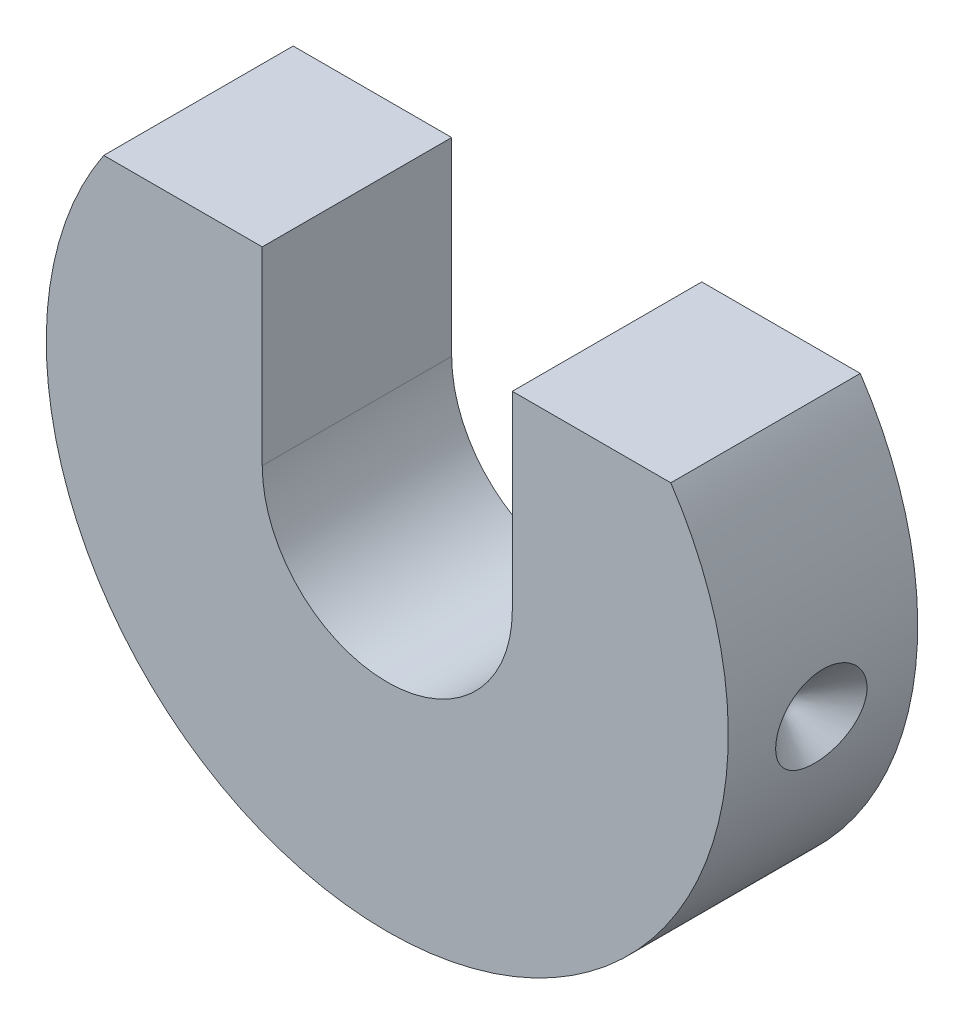
SolidWorks part; units mm, degrees
ref_plane "Front Plane" through (0, 0, 0) normal (0, 0, 1) x (1, 0, 0)
ref_plane "Top Plane" through (0, 0, 0) normal (0, 1, 0) x (1, 0, 0)
ref_plane "Right Plane" through (0, 0, 0) normal (1, 0, 0) x (0, 0, -1)
sketch "Sketch1" plane through (0, 0, 0) normal (0, 0, 1) x (1, 0, 0)
  line L0 (-14.9666, 10) -> (-6.6, 10)
  line L1 (-6.6, 0) -> (-6.6, 10)
  line L2 (6.6, 0) -> (6.6, 10)
  line L3 (6.6, 10) -> (14.9666, 10)
  arc A0 (-14.9666, 10) -> (14.9666, 10) centre (0, 0) ccw
  arc A1 (-6.6, 0) -> (6.6, 0) centre (0, 0) ccw
  dimension "D1" = 36
  dimension "D2" = 13.2
  dimension "D3" = 10
extrude "Boss-Extrude1" add sketch "Sketch1" along normal mid plane 10
sketch "Sketch2" plane through (0, 0, 0) normal (0, 0, 1) x (1, 0, 0)
  line L0 (-24.0476, -2) -> (21.912, -2) construction
  line L1 (18.8616, -5.3616) -> (18.8616, -2)
  line L2 (15.5, -2) -> (18.8616, -5.3616)
  line L3 (0, 0) -> (18, 0) construction
  line L4 (15.5, -2) -> (18.8616, -2)
  arc A0 (-14.9666, 10) -> (14.9666, 10) centre (0, 0) ccw construction
  dimension "D1" = 2
  dimension "D2" = 45
  dimension "D3" = 2.5
revolve "Cut-Revolve1" cut sketch "Sketch2" angle 360 about L0
mirror "Mirror1" about plane through (0, 0, 0) normal (1, 0, 0) of "Cut-Revolve1"
